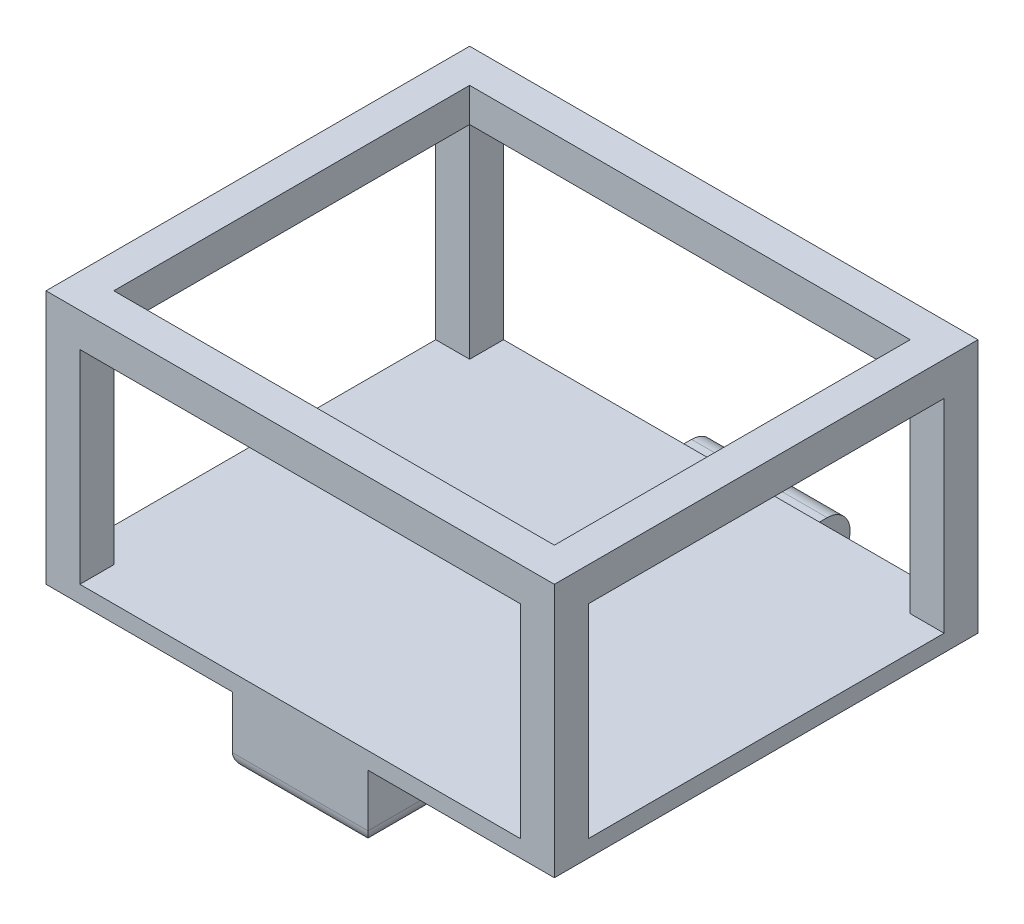
SolidWorks part; units mm, degrees
ref_plane "Front Plane" through (0, 0, 0) normal (0, 0, 1) x (1, 0, 0)
ref_plane "Top Plane" through (0, 0, 0) normal (0, 1, 0) x (1, 0, 0)
ref_plane "Right Plane" through (0, 0, 0) normal (1, 0, 0) x (0, 0, -1)
sketch "Sketch1" plane through (0, 0, 0) normal (0, 0, 1) x (1, 0, 0)
  line L1 (-400, 200) -> (400, 200)
  line L2 (-400, 200) -> (-400, -200)
  line L3 (-400, -200) -> (400, -200)
  line L4 (400, 200) -> (400, -200)
  line L5 (-400, 200) -> (400, -200) construction
  line L6 (-400, -200) -> (400, 200) construction
  point P0 (0, 0)
  dimension "D1" = 800
  dimension "D2" = 400
extrude "Boss-Extrude1" add sketch "Sketch1" along normal blind 12500
sketch "Sketch2" plane through (0, 200, 0) normal (0, 1, 0) x (1, 0, 0)
  line L0 (400, -12500) -> (-400, -12500) construction
  line L1 (-1500, -10000) -> (1500, -10000)
  line L2 (-1500, -10000) -> (-1500, -12500)
  line L3 (-1500, -12500) -> (1500, -12500)
  line L4 (1500, -10000) -> (1500, -12500)
  line L5 (-1500, -10000) -> (1500, -12500) construction
  line L6 (-1500, -12500) -> (1500, -10000) construction
  point P0 (0, -11250)
  dimension "D1" = 2500
  dimension "D2" = 3000
extrude "Boss-Extrude2" add sketch "Sketch2" along normal blind 1500
sketch "Sketch3" plane through (1500, 0, 0) normal (1, 0, 0) x (0, 0, -1)
  line L0 (-12500, 1700) -> (-10000, 1700) construction
  line L1 (-12300, 1500) -> (-10200, 1500)
  line L2 (-12300, 1500) -> (-12300, 300)
  line L3 (-12300, 300) -> (-10200, 300)
  line L4 (-10200, 1500) -> (-10200, 300)
  line L5 (-10000, 1700) -> (-10000, 200) construction
  line L6 (-12500, 1700) -> (-12500, 200) construction
  line L7 (-12500, 200) -> (-10000, 200) construction
  dimension "D1" = 200
  dimension "D2" = 200
  dimension "D3" = 200
  dimension "D4" = 100
extrude "Cut-Extrude1" cut sketch "Sketch3" against normal blind 3000
sketch "Sketch4" plane through (0, 0, 10000) normal (0, 0, -1) x (-1, 0, 0)
  line L0 (-1500, 1700) -> (1500, 1700) construction
  line L1 (-1300, 1500) -> (1300, 1500)
  line L2 (-1300, 1500) -> (-1300, 300)
  line L3 (-1300, 300) -> (1300, 300)
  line L4 (1300, 1500) -> (1300, 300)
  line L5 (-1500, 1700) -> (-1500, 200) construction
  line L6 (1500, 1700) -> (1500, 200) construction
  line L7 (400, 200) -> (1500, 200) construction
  dimension "D1" = 200
  dimension "D2" = 200
  dimension "D3" = 200
  dimension "D4" = 100
extrude "Cut-Extrude2" cut sketch "Sketch4" against normal blind 3000
sketch "Sketch5" plane through (0, 1700, 0) normal (0, 1, 0) x (1, 0, 0)
  line L0 (1500, -10000) -> (-1500, -10000) construction
  line L1 (-1300, -10200) -> (1300, -10200)
  line L2 (-1300, -10200) -> (-1300, -12300)
  line L3 (-1300, -12300) -> (1300, -12300)
  line L4 (1300, -10200) -> (1300, -12300)
  line L5 (-1500, -10000) -> (-1500, -12500) construction
  line L6 (-1500, -12500) -> (1500, -12500) construction
  line L7 (1500, -12500) -> (1500, -10000) construction
  dimension "D1" = 200
  dimension "D2" = 200
  dimension "D3" = 200
  dimension "D4" = 200
extrude "Cut-Extrude3" cut sketch "Sketch5" against normal blind 1000
fillet "Fillet1" radius 90 5 edges at (0, -200, 12500) (-400, -200, 6250) (400, 200, 5000) (-400, 200, 5000) (400, -200, 6250)
sketch "Sketch6" plane through (0, 0, 10000) normal (0, 0, -1) x (-1, 0, 0)
  line L1 (-909.8169, 692.8211) -> (721.4629, 692.8211)
  line L2 (-909.8169, 692.8211) -> (-909.8169, -289.3102)
  line L3 (-909.8169, -289.3102) -> (721.4629, -289.3102)
  line L4 (721.4629, 692.8211) -> (721.4629, -289.3102)
extrude "Cut-Extrude4" cut sketch "Sketch6" along normal through all
sketch "Sketch7" plane through (400, 0, 0) normal (1, 0, 0) x (0, 0, -1)
  line L0 (-10304.1329, 0) -> (-9790.2638, 0) construction
  line L1 (-10304.1329, 135.7121) -> (-9790.2638, 135.7121)
  line L2 (-10304.1329, -135.7121) -> (-9790.2638, -135.7121)
  arc A0 (-10304.1329, 135.7121) -> (-10304.1329, -135.7121) centre (-10304.1329, 0) ccw
  arc A1 (-9790.2638, -135.7121) -> (-9790.2638, 135.7121) centre (-9790.2638, 0) ccw
  point P3 (-10047.1984, 0)
extrude "Boss-Extrude3" add sketch "Sketch7" against normal up to surface (800 mm away) up to face at (-400, 45, 11250)
equation "\"‘\"=90"
